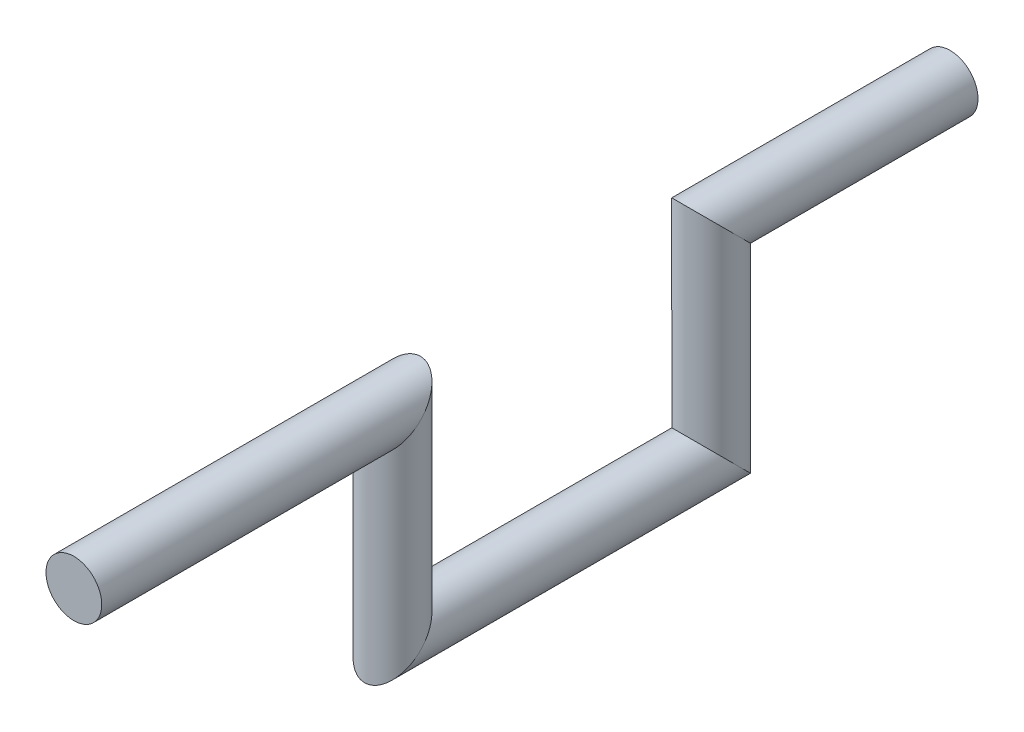
SolidWorks part; units mm, degrees
ref_plane "前视基准面" through (0, 0, 0) normal (0, 0, 1) x (1, 0, 0)
ref_plane "上视基准面" through (0, 0, 0) normal (0, 1, 0) x (1, 0, 0)
ref_plane "右视基准面" through (0, 0, 0) normal (1, 0, 0) x (0, 0, -1)
sketch "草图1" plane through (0, 0, 0) normal (0, 0, 1) x (1, 0, 0)
  circle A0 centre (0, 0) radius 7
  dimension "D1" = 14
sketch "草图3" plane through (0, 0, 0) normal (1, 0, 0) x (0, 0, -1)
  line L0 (0, 0) -> (80, 0)
  line L1 (80, 0) -> (80, -50)
  line L2 (80, -50) -> (160, -50)
  line L3 (160, -50) -> (160, 0)
  line L4 (160, 0) -> (220, 0)
  dimension "D1" = 80
  dimension "D2" = 80
  dimension "D3" = 60
  dimension "D4" = 50
sweep "扫描1" add profiles "草图1" path "草图3"
